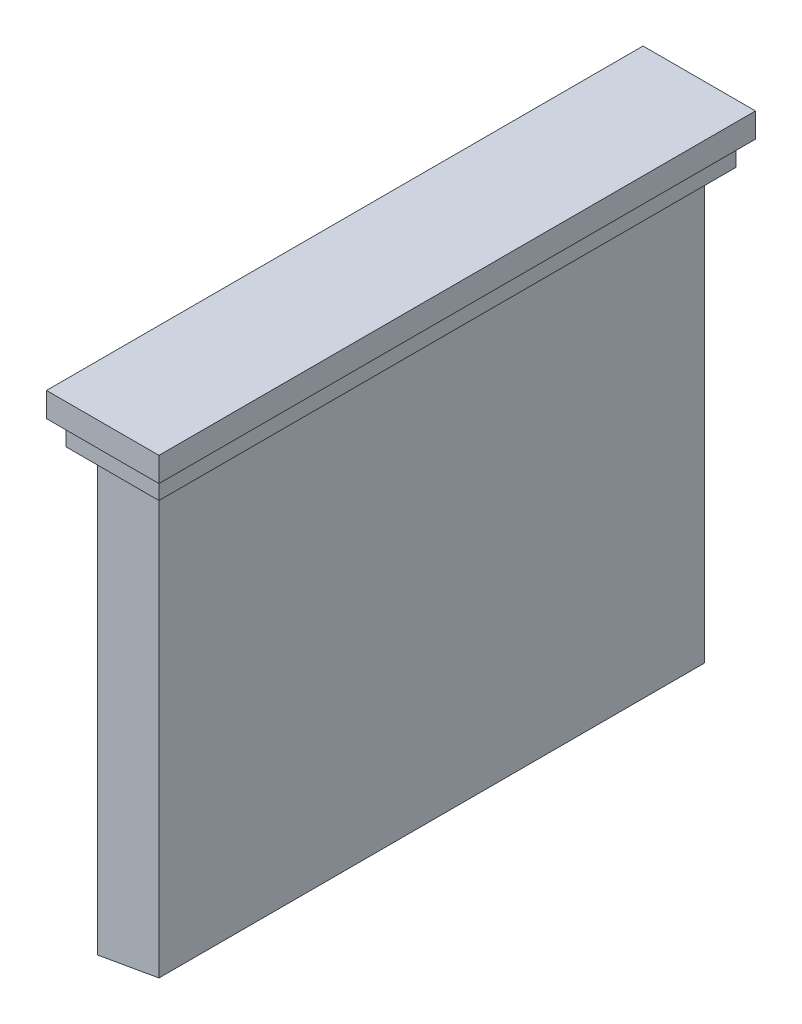
SolidWorks part; units mm, degrees
ref_plane "Front Plane" through (0, 0, 0) normal (0, 0, 1) x (1, 0, 0)
ref_plane "Top Plane" through (0, 0, 0) normal (0, 1, 0) x (1, 0, 0)
ref_plane "Right Plane" through (0, 0, 0) normal (1, 0, 0) x (0, 0, -1)
sketch "Sketch1" plane through (0, 0, 0) normal (0, 1, 0) x (1, 0, 0)
  line L4 (0, 0) -> (0, 13.6249) construction
  line L5 (0, 0) -> (16.3313, 0) construction
  line L6 (-3.14, 27.89) -> (3.14, 27.89)
  line L7 (3.14, 27.89) -> (3.14, -27.89)
  line L8 (-3.14, -27.89) -> (3.14, -27.89)
  line L9 (-3.14, 27.89) -> (-3.14, -27.89)
extrude "Boss-Extrude1" add sketch "Sketch1" along normal blind 45
sketch "Sketch2" plane through (0, 0, 27.89) normal (0, 0, 1) x (1, 0, 0)
  line L0 (-3.14, 0) -> (3.14, 0)
  line L2 (3.14, 0) -> (3.14, 1.1073)
  line L3 (3.14, 45) -> (3.14, 0) construction
  line L4 (3.14, 1.1073) -> (-3.14, 0)
  dimension "D1" = 10
extrude "Cut-Extrude1" cut sketch "Sketch2" against normal through all
sketch "Sketch3" plane through (0, 45, 0) normal (0, 1, 0) x (1, 0, 0)
  line L0 (-4.75, 29.5) -> (4.75, 29.5)
  line L5 (4.75, 29.5) -> (4.75, -29.5)
  line L6 (-4.75, -29.5) -> (4.75, -29.5)
  line L7 (-4.75, 29.5) -> (-4.75, -29.5)
extrude "Boss-Extrude2" add sketch "Sketch3" along normal blind 2.5
sketch "Sketch4" plane through (0, 47.5, 0) normal (0, 1, 0) x (1, 0, 0)
  line L0 (-5.75, 30.5) -> (5.75, 30.5)
  line L5 (5.75, 30.5) -> (5.75, -30.5)
  line L6 (-5.75, -30.5) -> (5.75, -30.5)
  line L7 (-5.75, 30.5) -> (-5.75, -30.5)
extrude "Boss-Extrude3" add sketch "Sketch4" along normal blind 2.5
